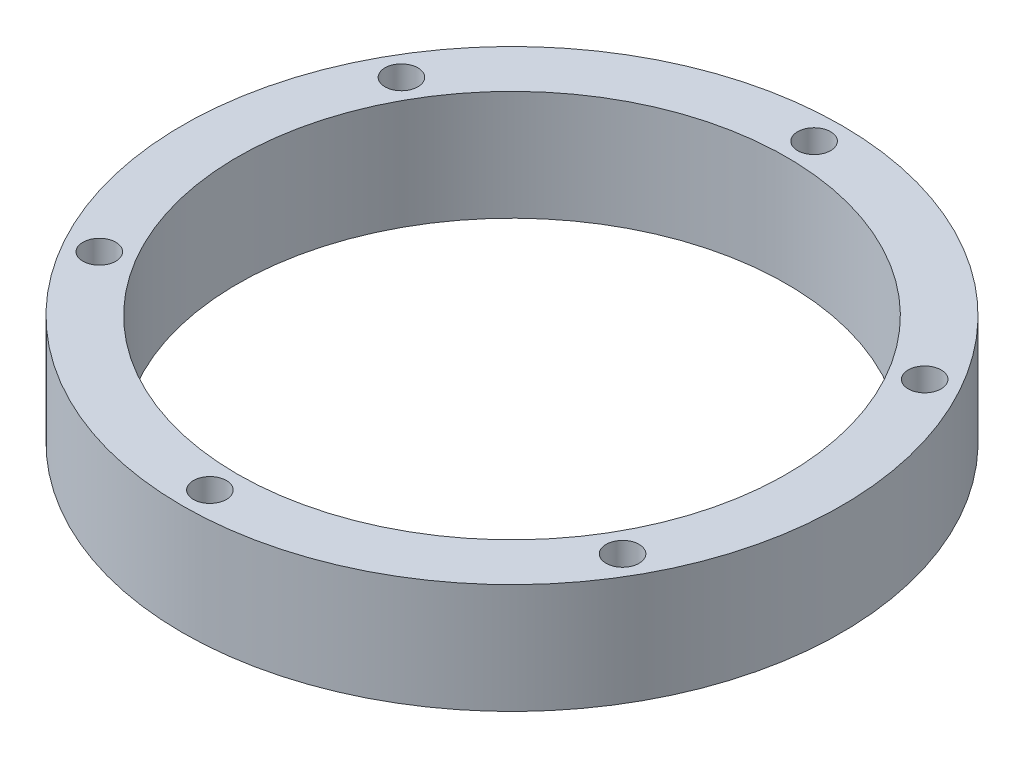
from build123d import *

# Parameters (mm, degrees)
SKETCH_1_R               = 60
SKETCH_1_R_2             = 50
EXTRUDE_1_DEPTH          = 20
SKETCH_2_R               = 3
CUT_EXTRUDE_1_DEPTH      = 88.177978871
PATTERN_CIRCULAR_1_COUNT = 6


with BuildPart() as part:
    # 草图1 → 凸台-拉伸1 (new body)
    with BuildSketch(Plane(origin=(0, 0, 0), x_dir=(1, 0, 0), z_dir=(0, 1, 0))):
        with Locations(Location((0, 0, 0), (0, 0, 270))):
            Circle(SKETCH_1_R)
        with Locations(Location((0, 0, 0), (0, 0, 270))):
            Circle(SKETCH_1_R_2, mode=Mode.SUBTRACT)
    extrude(amount=EXTRUDE_1_DEPTH)

    # 草图2 → 切除-拉伸1 (cut, through all)
    with BuildSketch(Plane(origin=(0, 20, 0), x_dir=(1, 0, 0), z_dir=(0, 1, 0))):
        with Locations(Location((0, 55, 0), (0, 0, 270))):
            Circle(SKETCH_2_R)
    cut_extrude_1 = extrude(amount=-CUT_EXTRUDE_1_DEPTH, mode=Mode.SUBTRACT)

    # 阵列(圆周)1: 切除-拉伸1 ×6 about axis
    pattern_circular_1_axis = Axis((0, 0, 0), (0, 1, 0))
    for i in range(1, PATTERN_CIRCULAR_1_COUNT):
        add(cut_extrude_1.rotate(pattern_circular_1_axis, i * 360 / PATTERN_CIRCULAR_1_COUNT), mode=Mode.SUBTRACT)


solid = part.part
